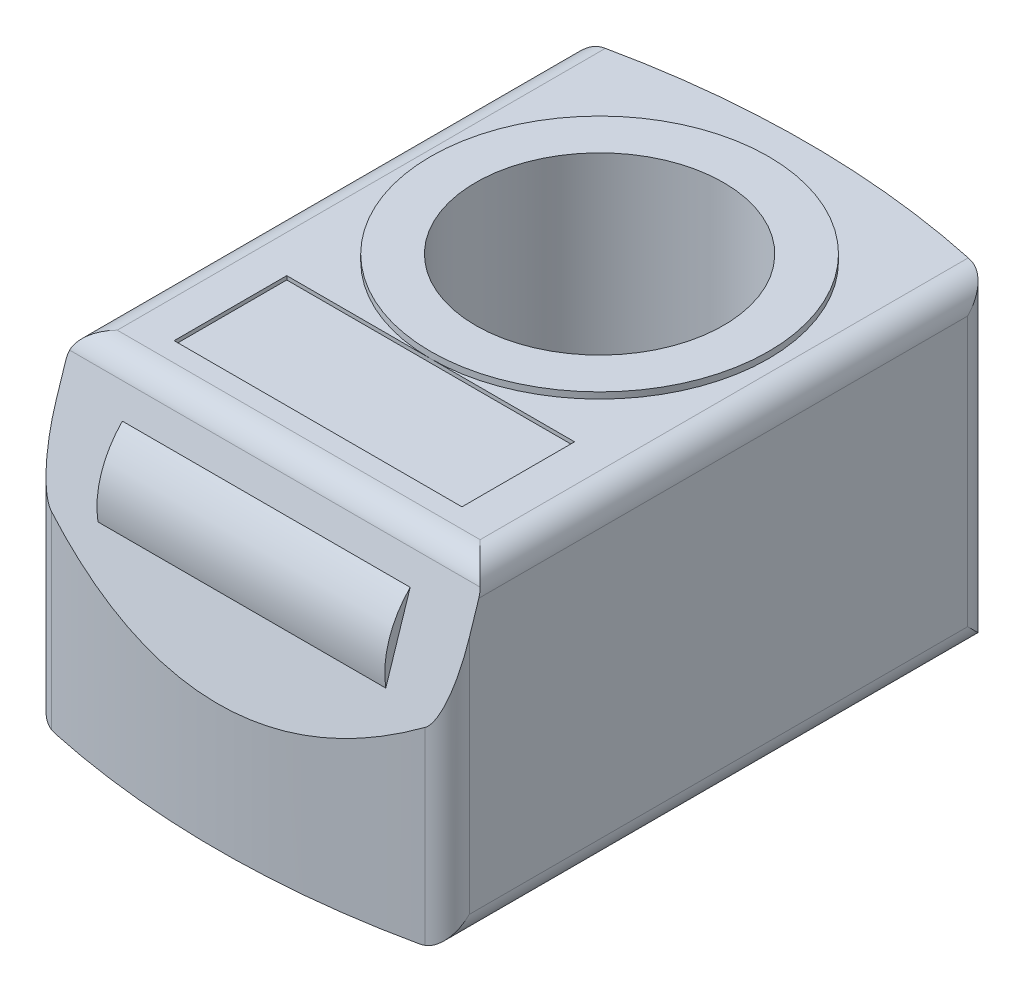
from build123d import *

# Parameters (mm, degrees)
EXTRUDE_1_DEPTH          = 20.5
EXTRUDE_START            = -3
EXTRUDE_2_DEPTH          = 3
EXTRUDE_START_2          = -2
EXTRUDE_3_DEPTH          = 2
CUT_EXTRUDE_1_DEPTH      = 35
CUT_EXTRUDE_1_DEPTH_BACK = 35
SKETCH_4_W               = 40
SKETCH_4_H               = 35
SKETCH_6_W               = 9.9
SKETCH_6_H               = 24
SKETCH_7_W               = 9.9
SKETCH_7_H               = 2
CUT_EXTRUDE_2_DEPTH      = 20
CUT_EXTRUDE_2_DEPTH_BACK = 20
SKETCH_8_W               = 3.6
SKETCH_8_H               = 1
SKETCH_10_W              = 1.5
SKETCH_10_H              = 5
EXTRUDE_4_DEPTH          = 11.5
EXTRUDE_4_DEPTH_BACK     = 11.5
SKETCH_12_W              = 23
SKETCH_12_H              = 9
CUT_EXTRUDE_3_DEPTH      = 0.3


with BuildPart() as part:
    # 草图1 → 凸台-拉伸1 (new body)
    with BuildSketch(Plane(origin=(0, -9, 0), x_dir=(-1, 0, 0), z_dir=(0, 1, 0))):
        with BuildLine():
            Line((16.5, -12.913670522), (16.5, 26.913670522))
            ThreePointArc((16.5, 26.913670522), (16.059625735, 28.165695908), (14.932432432, 28.866361535))
            ThreePointArc((14.932432432, 28.866361535), (0, 30.5), (-14.932432432, 28.866361535))
            ThreePointArc((-14.932432432, 28.866361535), (-16.059625735, 28.165695908), (-16.5, 26.913670522))
            Line((-16.5, 26.913670522), (-16.5, -12.913670522))
            ThreePointArc((-16.5, -12.913670522), (-16.059625735, -14.165695908), (-14.932432432, -14.866361535))
            ThreePointArc((-14.932432432, -14.866361535), (0, -16.5), (14.932432432, -14.866361535))
            ThreePointArc((14.932432432, -14.866361535), (16.059625735, -14.165695908), (16.5, -12.913670522))
        make_face()
    extrude(amount=EXTRUDE_1_DEPTH)

    # 草图2 → 凸台-拉伸2 (add)
    with BuildSketch(Plane(origin=(0, -9, 0), x_dir=(-1, 0, 0), z_dir=(0, 1, 0)).offset(EXTRUDE_START)):
        with BuildLine():
            Line((16.5, -12.913670522), (16.5, 26.913670522))
            ThreePointArc((16.5, 26.913670522), (16.059625735, 28.165695908), (14.932432432, 28.866361535))
            ThreePointArc((14.932432432, 28.866361535), (0, 30.5), (-14.932432432, 28.866361535))
            ThreePointArc((-14.932432432, 28.866361535), (-16.059625735, 28.165695908), (-16.5, 26.913670522))
            Line((-16.5, 26.913670522), (-16.5, -12.913670522))
            ThreePointArc((-16.5, -12.913670522), (-16.059625735, -14.165695908), (-14.932432432, -14.866361535))
            ThreePointArc((-14.932432432, -14.866361535), (0, -16.5), (14.932432432, -14.866361535))
            ThreePointArc((14.932432432, -14.866361535), (16.059625735, -14.165695908), (16.5, -12.913670522))
        make_face()
    extrude(amount=EXTRUDE_2_DEPTH)

    # 草图3 → 凸台-拉伸3 (add)
    with BuildSketch(Plane(origin=(0, -12, 0), x_dir=(-1, 0, 0), z_dir=(0, 1, 0)).offset(EXTRUDE_START_2)):
        with BuildLine():
            Line((16.5, -12.913670522), (16.5, 26.913670522))
            ThreePointArc((16.5, 26.913670522), (16.059625735, 28.165695908), (14.932432432, 28.866361535))
            ThreePointArc((14.932432432, 28.866361535), (0, 30.5), (-14.932432432, 28.866361535))
            ThreePointArc((-14.932432432, 28.866361535), (-16.059625735, 28.165695908), (-16.5, 26.913670522))
            Line((-16.5, 26.913670522), (-16.5, -12.913670522))
            ThreePointArc((-16.5, -12.913670522), (-16.059625735, -14.165695908), (-14.932432432, -14.866361535))
            ThreePointArc((-14.932432432, -14.866361535), (0, -16.5), (14.932432432, -14.866361535))
            ThreePointArc((14.932432432, -14.866361535), (16.059625735, -14.165695908), (16.5, -12.913670522))
        make_face()
    extrude(amount=EXTRUDE_3_DEPTH)

    # 草图4 → 切除-拉伸1 (cut, two sides: drawn at the far end of the back side and taken through both)
    with BuildSketch(Plane.XY.offset(-CUT_EXTRUDE_1_DEPTH_BACK)):
        with Locations((0, -2.5)):
            Rectangle(SKETCH_4_W, SKETCH_4_H)
        with BuildLine():
            Line((-16.5, 9.5), (-16.5, -12))
            ThreePointArc((-16.5, -12), (-15.914213562, -13.414213562), (-14.5, -14))
            Line((-14.5, -14), (14.5, -14))
            ThreePointArc((14.5, -14), (15.914213562, -13.414213562), (16.5, -12))
            Line((16.5, -12), (16.5, 9.5))
            ThreePointArc((16.5, 9.5), (15.914213562, 10.914213562), (14.5, 11.5))
            Line((14.5, 11.5), (-14.5, 11.5))
            ThreePointArc((-14.5, 11.5), (-15.914213562, 10.914213562), (-16.5, 9.5))
        make_face(mode=Mode.SUBTRACT)
    extrude(amount=CUT_EXTRUDE_1_DEPTH + CUT_EXTRUDE_1_DEPTH_BACK, mode=Mode.SUBTRACT)

    # 草图6 → 切除-旋转1 (revolve, cut)
    with BuildSketch(Plane(origin=(0, 0, 0), x_dir=(0, 0, -1), z_dir=(1, 0, 0))):
        with Locations((-4.95, 0)):
            Rectangle(SKETCH_6_W, SKETCH_6_H)
    revolve(axis=Axis((0, 12, 0), (0, -1, 0)), mode=Mode.SUBTRACT)

    # 草图7 → 切除-旋转2 (revolve, cut)
    with BuildSketch(Plane(origin=(0, 0, 0), x_dir=(0, 0, -1), z_dir=(1, 0, 0))):
        with Locations((-4.95, -13)):
            Rectangle(SKETCH_7_W, SKETCH_7_H)
    revolve(axis=Axis((0, -12, 0), (0, -1, 0)), mode=Mode.SUBTRACT)

    # 草图9 → 切除-拉伸2 (cut, two sides: drawn at the far end of the back side and taken through both)
    with BuildSketch(Plane(origin=(0, 0, 0), x_dir=(0, 0, -1), z_dir=(1, 0, 0)).offset(-CUT_EXTRUDE_2_DEPTH_BACK)):
        with BuildLine():
            Line((-35, -25), (-15, -25))
            Line((-15, -25), (-15, -14))
            Line((-15, -14), (-30.5, -14))
            Line((-30.5, -14), (-30.5, -3.888417686))
            Line((-30.5, -3.888417686), (-25.949027977, 10.118033989))
            ThreePointArc((-25.949027977, 10.118033989), (-25.222485449, 11.118033989), (-24.046914944, 11.5))
            Line((-24.046914944, 11.5), (-15, 11.5))
            Line((-15, 11.5), (-15, 25))
            Line((-15, 25), (-35, 25))
            Line((-35, 25), (-35, -25))
        make_face()
    extrude(amount=CUT_EXTRUDE_2_DEPTH + CUT_EXTRUDE_2_DEPTH_BACK, mode=Mode.SUBTRACT)

    # 草图8 → 旋转1 (revolve)
    with BuildSketch(Plane(origin=(0, 0, 0), x_dir=(0, 0, -1), z_dir=(1, 0, 0))):
        with Locations((-11.7, 11.5)):
            Rectangle(SKETCH_8_W, SKETCH_8_H)
    revolve(axis=Axis((0, 5, 0), (0, -1, 0)))

    # 草图5 → 旋转2 (revolve)
    with BuildSketch(Plane(origin=(0, 0, 0), x_dir=(0, 0, -1), z_dir=(1, 0, 0))):
        Polygon((-22, -17), (-24.7, -17), (-25, -16.7), (-25, -10), (-22, -10), align=None)
    revolve(axis=Axis((0, -10, 22), (0, -1, 0)))

    # 草图10 → 切除-旋转3 (revolve, cut)
    with BuildSketch(Plane(origin=(0, 0, 0), x_dir=(0, 0, -1), z_dir=(1, 0, 0)), mode=Mode.PRIVATE) as cut_revolve_3_sk:
        with Locations((-21.25, -14.5)):
            Rectangle(SKETCH_10_W, SKETCH_10_H)
    revolve(cut_revolve_3_sk.sketch.rotate(Axis((0, -17, 22), (0, 1, 0)), 180), axis=Axis((0, -17, 22), (0, 1, 0)), mode=Mode.SUBTRACT)

    # 草图11 → 凸台-拉伸4 (add, two sides: drawn at the far end of the back side and taken through both)
    with BuildSketch(Plane(origin=(0, 0, 0), x_dir=(0, 0, -1), z_dir=(1, 0, 0)).offset(-EXTRUDE_4_DEPTH_BACK)):
        with BuildLine():
            Line((-28.586737114, 2), (-26, 2))
            Line((-26, 2), (-26, 8))
            Line((-26, 8), (-26.637218937, 8))
            ThreePointArc((-26.637218937, 8), (-28.326233362, 5.232075627), (-28.586737114, 2))
        make_face()
    extrude(amount=EXTRUDE_4_DEPTH + EXTRUDE_4_DEPTH_BACK)

    # 草图12 → 切除-拉伸3 (cut)
    with BuildSketch(Plane(origin=(0, 11.5, 0), x_dir=(-1, 0, 0), z_dir=(0, 1, 0))):
        with Locations((0, 18)):
            Rectangle(SKETCH_12_W, SKETCH_12_H)
    extrude(amount=-CUT_EXTRUDE_3_DEPTH, mode=Mode.SUBTRACT)


solid = part.part
